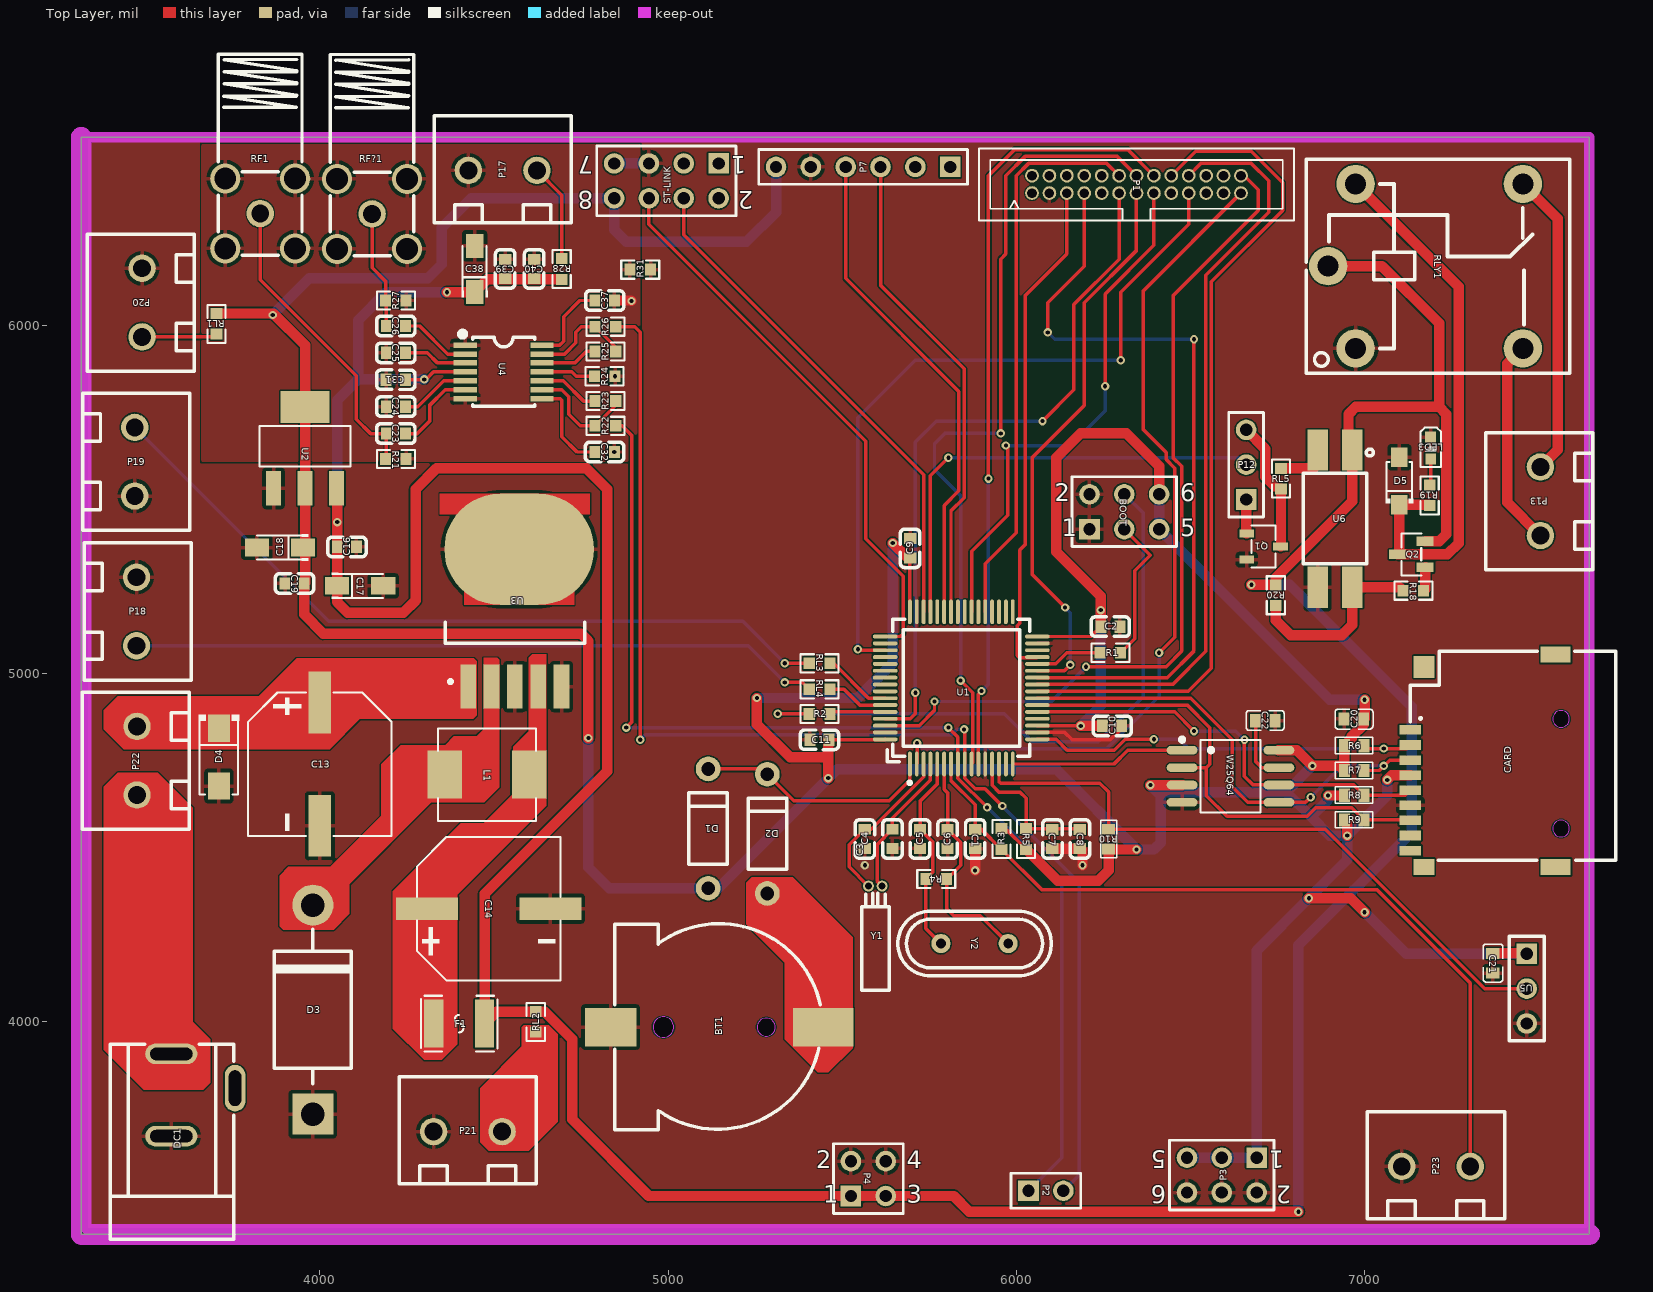
[diagram p0: Top Layer view]
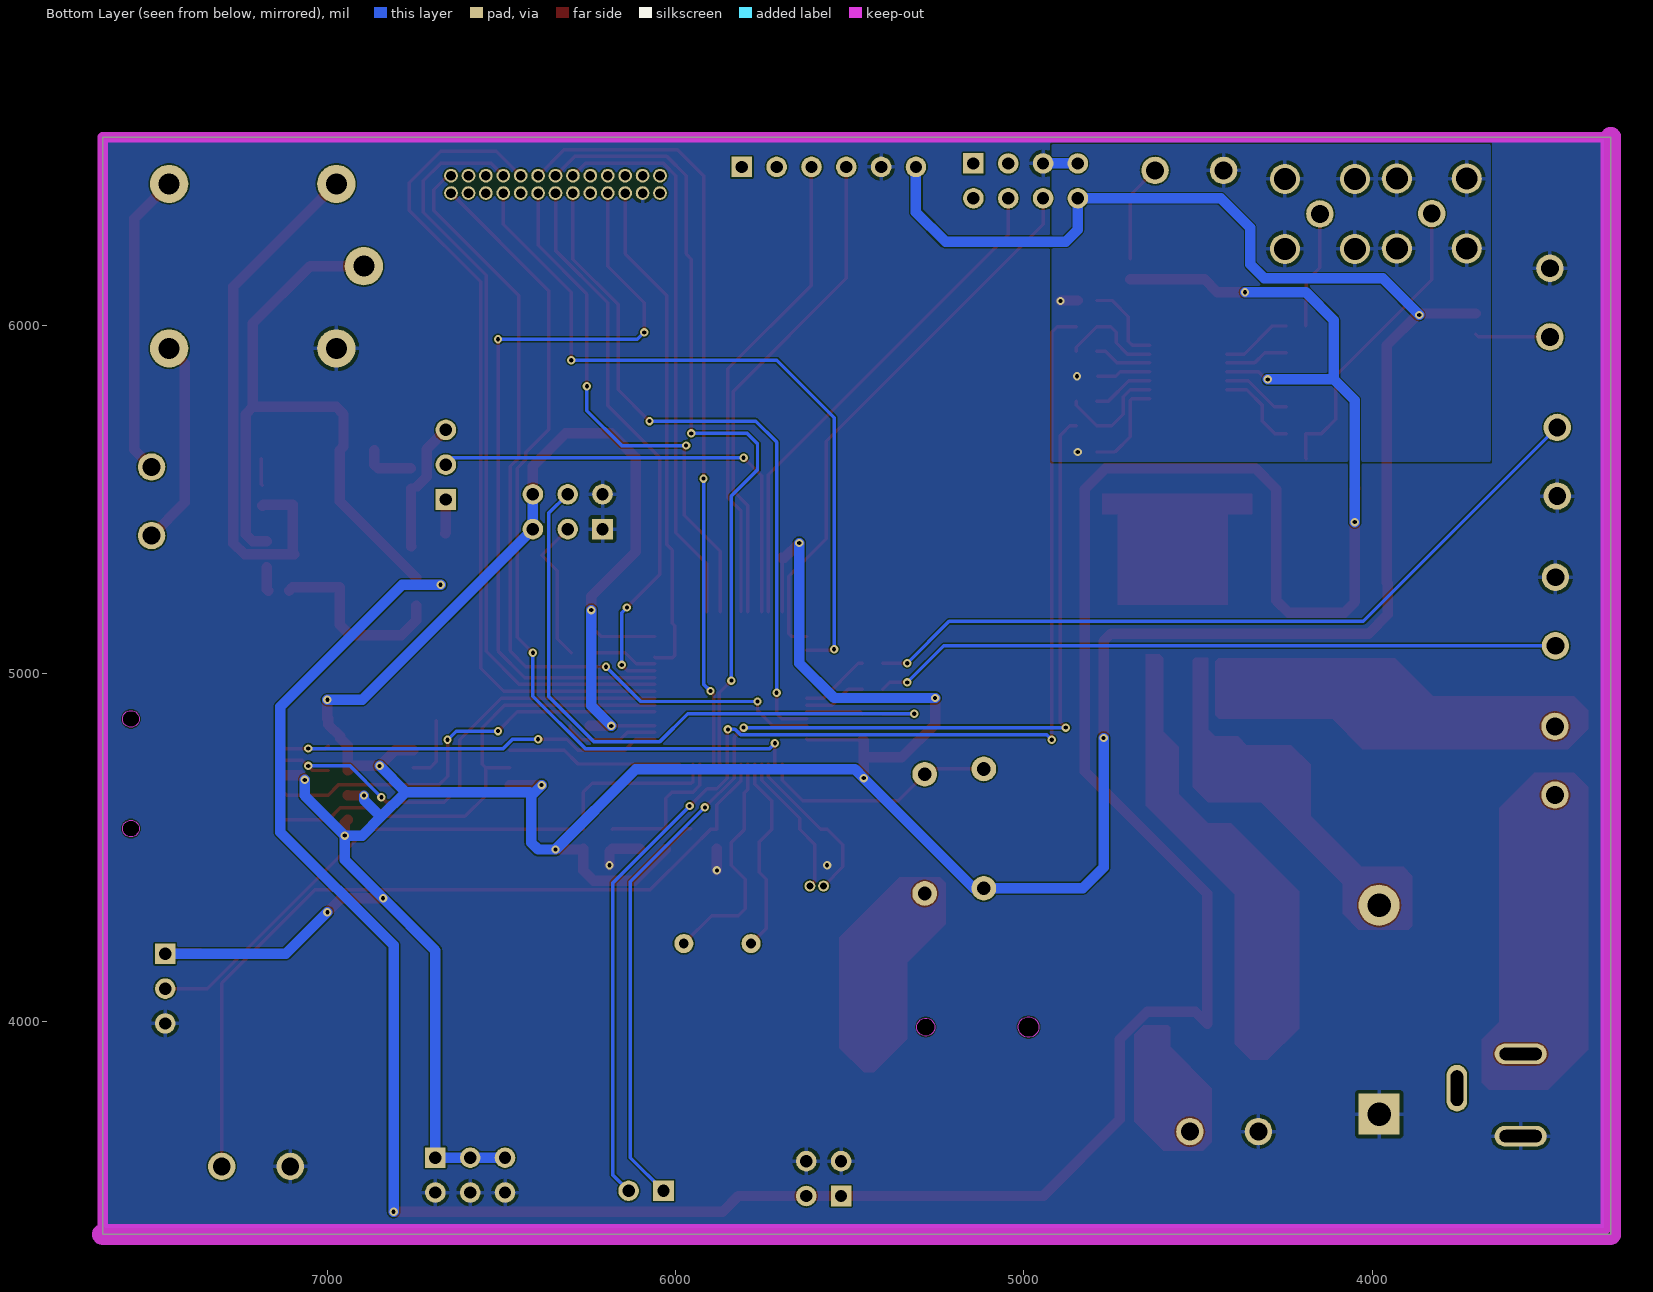
[diagram p1: Bottom Layer view, seen from below]
# Altium PCB MISC51485.pcbdoc
Units mil, origin at the board's own origin, x right, y up, seen from the top; angles counter-clockwise.
Board outline 4330.71 x 3150 mil, 2 copper layers (Top Layer, Bottom Layer); 98 components, 109 nets, 353 pads, 61 vias.

## Layer stack, top to bottom (the 12.6 mil dielectric is the usual default, probably not edited)
Top Solder Mask Layer: solder mask 0.4, Solder Resist, Dk 3.5
Top Layer: signal copper 1.4
Dielectric 1: surface 12.6, FR-4, Dk 4.8
Bottom Layer: signal copper 1.4
Bottom Solder Mask Layer: solder mask 0.4, Solder Resist, Dk 3.5

## Board outline
7645,3390 3315,3390 3315,6540 7645.71,6540 7645,6539.61

## Design rules (kind name [scope] priority, off if disabled: settings)
BoardOutlineClearance Clearance_1 [All] p2: genericclearance=4 ignorepadtopadclearanceinfootprint=FALSE except(0: Hole-OutlineEdge Arc-SplitContinuation Track-SplitContinuation SMDPad-SplitContinuation THPad-SplitContinuation Via-SplitContinuation Fill-SplitContinuation Region-SplitContinuation Poly-SplitContinuation Text-SplitContinuation Hole-SplitContinuation; 4: Arc-OutlineEdge Track-OutlineEdge SMDPad-OutlineEdge THPad-OutlineEdge Via-OutlineEdge Fill-OutlineEdge Region-OutlineEdge Poly-OutlineEdge Text-OutlineEdge Arc-CutoutEdge Track-CutoutEdge SMDPad-CutoutEdge THPad-CutoutEdge Poly-CutoutEdge; 6: Via-CutoutEdge Fill-CutoutEdge Region-CutoutEdge Text-CutoutEdge; 6.9: Hole-CutoutEdge)
Clearance [All] p1: gap=4 ignorepadtopadclearanceinfootprint=FALSE except(0: Hole-Track Hole-SMDPad Hole-THPad Hole-Via Fill-Hole Region-Hole Poly-Hole Hole-Arc Hole-Text)
DiffPairsRouting [All] p1: maxlimit=10 minlimit=6 mostfreqgap=6 toplayer_minwidth=15 toplayer_prefwidth=15 toplayer_maxwidth=15 toplayer_mingap=10 toplayer_prefgap=10 toplayer_maxgap=10 bottomlayer_minwidth=15 bottomlayer_prefwidth=15 bottomlayer_maxwidth=15 bottomlayer_mingap=10 bottomlayer_prefgap=10 bottomlayer_maxgap=10 maxuncoupledlength=10
HoleToHoleClearance ComponentClearance [All] p1: gap=10 allowstackedmicrovias=TRUE
Length netLength [All] p1: minlimit=0 maxlimit=0
MatchedLengths netLengthTolerance [All] p1: tolerance=1000
PolygonConnect [(InNet('AGND') OR InNet('GND'))] p1: connectstyle=Relief reliefconductorwidth=10 reliefentries=4 polygonreliefangle="90 Angle" airgapwidth=10 via.connectstyle=Relief via.reliefconductorwidth=10 via.reliefentries=4 via.polygonreliefangle="90 Angle" via.airgapwidth=10
RoutingVias [All] p1: holewidth=12 width=24 viastyle="Through Hole" minholewidth=1 minwidth=1 maxholewidth=28 maxwidth=50
SolderMaskExpansion [All] p1: expansion=4 istentingtop=FALSE
Width [All] p1: maxlimit=10 minlimit=10 preferedwidth=10 toplayer_minwidth=10 toplayer_maxwidth=300 toplayer_prefwidth=10 bottomlayer_minwidth=10 bottomlayer_maxwidth=300 bottomlayer_prefwidth=10
2 further rules are at their usual default settings.

## Components (designator, comment, footprint, x,y, rotation, side; value= is the part's Value field where it differs from the comment)
BOOT "Header 3X2" HDR2X3 6210,5415 r0 top
BT1 "BS-12-B3AA003" BAT-SMD_BS-12-B3AA011 5140,3985 r180 top
C1 "104" C0603 5881.72,4525 r270 top
C2 "104" C0603 6270,5135 r0 top
C3 "12pF" C0603 5644.23,4525.61 r90 top
C4 "12pF" C0603 5565,4525.61 r90 top
C5 "22pF" C0603 5723.46,4525.61 r90 top
C6 "22pF" C0603 5802.48,4525 r90 top
C7 "10uF" C0603 6103.2,4525 r270 top
C8 "104" C0603 6182.44,4525 r270 top
C9 "104" C0603 5695,5360 r90 top
C10 "104" C0603 6275,4850 r180 top
C11 "104" C0603 5435,4810 r0 top
C13 "GVM1V681M1010" CAP-SMD_BD10.0-L10.3-W10.3-LS10.9-FD 4000,4740 r270 top
C14 "EEEFK1V331P" CAP-SMD_BD10.0-L10.3-W10.3-FD 4485,4325 r0 top
C16 "104" C0603 4077.56,5363.94 r180 top
C17 "TAJA106K016RNJ" CAP-SMD_L3.2-W1.6-RD-C7171 4115.75,5252.05 r0 top
C18 "TAJA106K016RNJ" CAP-SMD_L3.2-W1.6-RD-C7171 3885.75,5362.17 r180 top
C19 "104" C0603 3927.56,5258.94 r0 top
C20 "Cap" CAP[0603] 6969.26,4869.85 r180 top
C21 "Cap" CAP[0603] 7368.1,4168.36 r270 top
C22 "Cap" CAP[0603] 6715,4865 r0 top
C23 "102" C0603 4218.55,5689.48 r0 top
C24 "102" C0603 4218.55,5766.66 r0 top
C25 "102" C0603 4218.55,5921.03 r0 top
C26 "102" C0603 4218.55,5998.21 r0 top
C31 "100pF" C0603 4217.94,5844.06 r180 top
C32 "0.1uF" C0603 4817.94,5636.45 r0 top
C37 "0.1uF" C0603 4817.94,6071.45 r180 top
C38 "10uF" CAP-SMD_L3.2-W1.6-RD-C7171 4444.5,6162.01 r90 top
C39 "0.1uF" C0603 4532.1,6161.7 r270 top
C40 "0.1uF" C0603 4615.28,6161.7 r270 top
CARD "TF PUSH" TF-SMD_TF-PUSH 7339.85,4749.85 r90 top
D1 "1N4733A_C5157516" DO-41_BD2.4-L4.7-P8.70-D0.9-RD 5115,4555 r270 top
D2 "1N4733A_C5157516" DO-41_BD2.4-L4.7-P8.70-D0.9-RD 5285,4540 r270 top
D3 "1N5822" DO-201AD_BD5.3-L8.4-P12.50-D1.4-FD 3980,4035 r90 top
D4 "1N4007_C727081" SMA_L4.3-W2.5-LS5.0-RD 3710,4760 r270 top
D5 "1N4007W" SOD-123FL_L2.7-W1.8-LS3.8-RD 7099.9,5553.14 r90 top
DC1 "DC-005-20A_C136744" DC-IN-TH_DC-005-20A 3665,3790 r90 top
F1 "BSMD1812-150-33V" F1812 4400,3995 r180 top
L1 "FXL0650-330-M" IND-SMD_L7.0-W6.6_FXL0650 4480,4710 r180 top
LED3 "NCD0603R1_C84263" LED0603-RD_RED 7189.87,5647.91 r270 top
P1 "X1270WV-2x13A-6TV01" IDC-TH_X1270WV-2X13A-6TV01 6345,6405 r0 top
P2 "Header 2" HDR1X2 6035,3515 r0 top
P3 "Header 3X2" HDR2X3 6690,3610 r180 top
P4 "Header 2X2" HDR2X2 5525,3500 r0 top
P7 "Header 6" HDR1X6 5810,6455 r180 top
P12 "Header 3" HDR1X3 6660,5500 r90 top
P13 "WJ126V-5.0-2P" CONN-TH_WJ126V-5.0-2P 7505,5495 r180 top
P17 "WJ126V-5.0-2P" CONN-TH_WJ126V-5.0-2P 4525,6445 r90 top
P18 "WJ126V-5.0-2P" CONN-TH_WJ126V-5.0-2P 3473.59,5178.49 r0 top
P19 "WJ126V-5.0-2P" CONN-TH_WJ126V-5.0-2P 3468.59,5608.49 r0 top
P20 "WJ126V-5.0-2P" CONN-TH_WJ126V-5.0-2P 3489.47,6065.51 r180 top
P21 "WJ126V-5.0-2P" CONN-TH_WJ126V-5.0-2P 4425,3685 r90 top
P22 "WJ126V-5.0-2P" CONN-TH_WJ126V-5.0-2P 3475,4750 r180 top
P23 "WJ126V-5.0-2P" CONN-TH_WJ126V-5.0-2P 7205,3585 r90 top
Q1 "DTC143ECA" SOT-23-3_L2.9-W1.6-P1.90-LS2.8-BR 6710,5365 r180 top
Q2 "MMBT3906" SOT-23-3_L2.9-W1.3-P1.90-LS2.4-BR 7134.21,5342.45 r0 top
R1 "10k" "R0603 - duplicate" 6270,5060 r0 top
R2 "10k" R0603 5435,4884.44 r0 top
R3 "10k" R0603 5957,4525.31 r90 top
R4 "1M" R0603 5770,4410 r180 top
R5 "10R" R0603 6028.13,4525.31 r270 top
R6 "Res" RES[0603] 6969.85,4792.85 r0 top
R7 "Res" RES[0603] 6969.85,4721.85 r0 top
R8 "Res" RES[0603] 6969.85,4650.85 r0 top
R9 "Res" RES[0603] 6969.85,4579.85 r0 top
R10 "Res" RES[0603] 6265,4525 r270 top
R18 "10k" "R0603 - duplicate" 7139.9,5238.14 r0 top
R19 "10k" "R0603 - duplicate" 7186.98,5511.83 r270 top
R20 "10k" "R0603 - duplicate" 6745,5225 r270 top
R21 "52.3R" R0603 4218.24,5616.45 r0 top
R22 "0" R0603 4820,5711.73 r180 top
R23 "100" R0603 4820,5782.84 r180 top
R24 "1K" R0603 4817.94,5853.95 r180 top
R25 "100" R0603 4820,5925.07 r180 top
R26 "0" R0603 4820,5996.18 r180 top
R27 "52.3R" R0603 4218.24,6071.45 r180 top
R28 "1K" R0603 4694.5,6162.01 r270 top
R31 "0" R0603 4920,6160 r180 top
RF1 "BWSMA-KWE-Z001" SMA-TH_BWSMA-KWE-Z001 3828.77,6321.23 r90 top
RF?1 "BWSMA-KWE-Z001" SMA-TH_BWSMA-KWE-Z001 4150,6320 r90 top
RL1 "330" "R0603 - duplicate" 3703.03,6004.51 r270 top
RL2 "330" "R0603 - duplicate" 4620,4000 r270 top
RL3 "330" "R0603 - duplicate" 5435,5029.72 r0 top
RL4 "330" "R0603 - duplicate" 5435,4955 r0 top
RL5 "330" "R0603 - duplicate" 6760,5560 r90 top
RLY1 "SRD-05VDC-SL-C" RELAY-TH_SRD-XXVDC-XL-C 7175,6170 r0 top
ST-LINK "Header 4X2" HDR2X4 5145,6465 r180 top
U1 "STM32F103RCT6" TQFP-64_L10.0-W10.0-P0.50-LS12.0-BL 5841.93,4959 r0 top
U2 "LM1117MPX-3.3/NOPB" SOT-223-3_L6.5-W3.4-P2.30-LS7.0-BR 3957.56,5648.94 r270 top
U3 "LM2596SX-5.0/NOPB" TO-263-5_L10.2-W8.9-P1.70-TL 4560,5160 r90 top
U4 "AD8302ARUZ-RL7" TSSOP-14_L5.0-W4.4-P0.65-LS6.4-BL 4527.94,5866.45 r270 top
U5 "DS18B20" H2.54-1X3(RM) 7465.79,4195.49 r270 top
U6 "BPC-817SC" OPTO-SMD-4_L4.6-W6.5-P2.54-LS10.3-BR 6915,5445 r90 top
W25Q64 "W25Q64JVSSIQ" SOIC-8_L5.3-W5.3-P1.27-LS8.0-BL 6615,4705.27 r270 top
Y1 "32.768kHz" OSC-TH_BD2.0-P0.70-D0.3 5595,4390 r90 top
Y2 "8MHz" OSC-TH_L11.1-W4.7-P4.88 5880,4225 r0 top

## Footprints (in the part's own frame and the unit in brackets; to place one, negate y for a bottom-side part, rotate by r counter-clockwise, add the part's x,y. Pads: shape width x height; smd on the part's side, far side on the other; paste and mask are expansions set on the pad)
BAT-SMD_BS-12-B3AA011 [mm]
  rect 3.75x2.8 smd: 1(7.75,0)
  rect 4.4x2.8 smd: 2(-7.75,0)
  Board Outline Layer lines w0.003: 4.649,0.098 4.65,0 4.649,-0.098 4.596,-0.287 4.497,-0.456 4.358,-0.594 4.187,-0.691 3.998,-0.741 3.802,-0.741 3.613,-0.691 3.443,-0.594 3.303,-0.456 3.204,-0.287 3.151,-0.098 3.15,0 3.151,0.098 3.204,0.287 3.303,0.456 3.443,0.594 3.613,0.691 3.802,0.741 3.998,0.741 4.188,0.691 4.358,0.594 4.497,0.456 4.596,0.287 4.649,0.098 ; -2.95,0.086 -2.95,0 -2.95,-0.086 -2.994,-0.251 -3.08,-0.399 -3.201,-0.52 -3.349,-0.606 -3.515,-0.65 -3.686,-0.65 -3.851,-0.606 -3.999,-0.52 -4.12,-0.399 -4.206,-0.251 -4.25,-0.086 -4.25,0 -4.25,0.086 -4.206,0.251 -4.12,0.399 -3.999,0.52 -3.851,0.606 -3.686,0.65 -3.514,0.65 -3.349,0.606 -3.201,0.52 -3.08,0.399 -2.994,0.251 -2.95,0.086
  Board Outline Layer region: -2.95,0 -2.95,0.086 -2.994,0.251 -3.08,0.399 -3.201,0.52 -3.349,0.606 -3.514,0.65 -3.686,0.65 -3.851,0.606 -3.999,0.52 -4.12,0.399 -4.206,0.251 -4.25,0.086 -4.25,0 -4.25,-0.086 -4.206,-0.251 -4.12,-0.399 -3.999,-0.52 -3.851,-0.606 -3.686,-0.65 -3.515,-0.65 -3.349,-0.606 -3.201,-0.52 -3.08,-0.399 -2.994,-0.251 -2.95,-0.086 -2.95,0 -2.95,0
  Board Outline Layer region: -2.95,0 -2.95,0.086 -2.994,0.251 -3.08,0.399 -3.201,0.52 -3.349,0.606 -3.514,0.65 -3.686,0.65 -3.851,0.606 -3.999,0.52 -4.12,0.399 -4.206,0.251 -4.25,0.086 -4.25,0 -4.25,-0.086 -4.206,-0.251 -4.12,-0.399 -3.999,-0.52 -3.851,-0.606 -3.686,-0.65 -3.515,-0.65 -3.349,-0.606 -3.201,-0.52 -3.08,-0.399 -2.994,-0.251 -2.95,-0.086 -2.95,0 -2.95,0
  Board Outline Layer region: -2.95,0 -2.95,0.086 -2.994,0.251 -3.08,0.399 -3.201,0.52 -3.349,0.606 -3.514,0.65 -3.686,0.65 -3.851,0.606 -3.999,0.52 -4.12,0.399 -4.206,0.251 -4.25,0.086 -4.25,0 -4.25,-0.086 -4.206,-0.251 -4.12,-0.399 -3.999,-0.52 -3.851,-0.606 -3.686,-0.65 -3.515,-0.65 -3.349,-0.606 -3.201,-0.52 -3.08,-0.399 -2.994,-0.251 -2.95,-0.086 -2.95,0 -2.95,0
  Board Outline Layer region: 4.65,0 4.649,0.098 4.596,0.287 4.497,0.456 4.358,0.594 4.188,0.691 3.998,0.741 3.802,0.741 3.613,0.691 3.443,0.594 3.303,0.456 3.204,0.287 3.151,0.098 3.15,0 3.151,-0.098 3.204,-0.287 3.303,-0.456 3.443,-0.594 3.613,-0.691 3.802,-0.741 3.998,-0.741 4.187,-0.691 4.358,-0.594 4.497,-0.456 4.596,-0.287 4.649,-0.098 4.65,0
  Board Outline Layer region: 4.65,0 4.649,0.098 4.596,0.287 4.497,0.456 4.358,0.594 4.188,0.691 3.998,0.741 3.802,0.741 3.613,0.691 3.443,0.594 3.303,0.456 3.204,0.287 3.151,0.098 3.15,0 3.151,-0.098 3.204,-0.287 3.303,-0.456 3.443,-0.594 3.613,-0.691 3.802,-0.741 3.998,-0.741 4.187,-0.691 4.358,-0.594 4.497,-0.456 4.596,-0.287 4.649,-0.098 4.65,0
  Board Outline Layer region: 4.65,0 4.649,0.098 4.596,0.287 4.497,0.456 4.358,0.594 4.188,0.691 3.998,0.741 3.802,0.741 3.613,0.691 3.443,0.594 3.303,0.456 3.204,0.287 3.151,0.098 3.15,0 3.151,-0.098 3.204,-0.287 3.303,-0.456 3.443,-0.594 3.613,-0.691 3.802,-0.741 3.998,-0.741 4.187,-0.691 4.358,-0.594 4.497,-0.456 4.596,-0.287 4.649,-0.098 4.65,0
  Multi-Layer board cut-out: -2.95,0 -2.95,0.086 -2.994,0.251 -3.08,0.399 -3.201,0.52 -3.349,0.606 -3.514,0.65 -3.686,0.65 -3.851,0.606 -3.999,0.52 -4.12,0.399 -4.206,0.251 -4.25,0.086 -4.25,0 -4.25,-0.086 -4.206,-0.251 -4.12,-0.399 -3.999,-0.52 -3.851,-0.606 -3.686,-0.65 -3.515,-0.65 -3.349,-0.606 -3.201,-0.52 -3.08,-0.399 -2.994,-0.251 -2.95,-0.086 -2.95,0 -2.95,0
  Multi-Layer board cut-out: 4.65,0 4.649,0.098 4.596,0.287 4.497,0.456 4.358,0.594 4.188,0.691 3.998,0.741 3.802,0.741 3.613,0.691 3.443,0.594 3.303,0.456 3.204,0.287 3.151,0.098 3.15,0 3.151,-0.098 3.204,-0.287 3.303,-0.456 3.443,-0.594 3.613,-0.691 3.802,-0.741 3.998,-0.741 4.187,-0.691 4.358,-0.594 4.497,-0.456 4.596,-0.287 4.649,-0.098 4.65,0
  silkscreen extent -7.55,-7.54 7.44,7.49
C0603 [mm]
  rect 0.8x0.9 smd paste+0 mask+0.051: 1(-0.7,0) 2(0.7,0)
  silkscreen extent -1.41,-0.71 1.39,0.72
CAP-SMD_BD10.0-L10.3-W10.3-FD [mm]
  rect 4.5x1.65 smd: 1(-4.5,0) 2(4.5,0)
  silkscreen extent -5.23,-5.23 5.23,5.23
CAP-SMD_BD10.0-L10.3-W10.3-LS10.9-FD [mm]
  rect 4.5x1.65 smd: 1(-4.5,0) 2(4.5,0)
  silkscreen extent -5.23,-5.23 5.23,5.23
CAP-SMD_L3.2-W1.6-RD-C7171 [mil]
  rect 69.19x51.02 smd: 1(-66.39,0) 2(66.39,0)
  silkscreen extent -81,-37 66,37
CAP[0603] [mm]
  rect 0.8x0.965 smd: 1(-0.716,0) 2(0.716,0)
  silkscreen extent -1.4,-0.71 1.37,0.74
CONN-TH_WJ126V-5.0-2P [mm]
  round 2 hole 1.3: 1(0,2.501) 2(0,-2.501)
  silkscreen extent -3.8,-5 4,5
DC-IN-TH_DC-005-20A [mm]
  oval 1.5x3.8 hole 0.9 slot 3.1 at 90 deg copper offset 0.001,0 paste+0 mask+0.051: 1(2.999,2.325)
  oval 1.5x3.8 hole 0.9 slot 3.1 at 90 deg copper offset 0,0 paste+0 mask+0.051: 2(-3.001,2.325)
  oval 3.4x1.5 hole 0.9 slot 2.6 at 0 deg copper offset 0.001,0 paste+0 mask+0.051: 3(0.5,-2.326)
  silkscreen extent -10.51,-2.24 3.71,6.78
DO-41_BD2.4-L4.7-P8.70-D0.9-RD [mm]
  round 1.8 hole 1: 1(-4.35,0) 2(4.35,0)
  silkscreen extent -2.6,-1.4 2.6,1.4
DO-201AD_BD5.3-L8.4-P12.50-D1.4-FD [mm]
  rect 3x3 hole 1.7: 1(-7.62,0)
  round 3 hole 1.7: 2(7.62,0)
  silkscreen extent -5.39,-2.8 5.87,2.8
F1812 [mil]
  rect 55.38x137.76 smd paste-3937.01 mask+2: 1(-72.97,0) 2(72.97,0)
  silkscreen extent -110,-80 110,80
H2.54-1X3(RM) [mm]
  rect 1.5x1.5 hole 0.9: 1(0,0)
  round 1.5 hole 0.9: 2(2.54,0) 3(5.08,0)
  silkscreen extent -1.27,-1.27 6.35,1.27
HDR1X2 [mm]
  rect 1.5x1.5 hole 0.9: 1(0,0)
  round 1.5 hole 0.9: 2(2.54,0)
  silkscreen extent -1.27,-1.27 3.81,1.27
HDR1X3 [mm]
  rect 1.5x1.5 hole 0.9: 1(0,0)
  round 1.5 hole 0.9: 2(2.54,0) 3(5.08,0)
  silkscreen extent -1.27,-1.27 6.35,1.27
HDR1X6 [mm]
  rect 1.5x1.5 hole 0.9: 1(0,0)
  round 1.5 hole 0.9: 2(2.54,0) 3(5.08,0) 4(7.62,0) 5(10.16,0) 6(12.7,0)
  silkscreen extent -1.27,-1.27 13.97,1.27
HDR2X2 [mm]
  rect 1.5x1.5 hole 0.9: 1(0,0)
  round 1.5 hole 0.9: 2(0,2.54) 3(2.54,0) 4(2.54,2.54)
  silkscreen extent -1.27,-1.27 3.81,3.81
HDR2X3 [mm]
  rect 1.5x1.5 hole 0.9: 1(0,0)
  round 1.5 hole 0.9: 2(0,2.54) 3(2.54,0) 4(2.54,2.54) 5(5.08,0) 6(5.08,2.54)
  silkscreen extent -1.27,-1.27 6.35,3.81
HDR2X4 [mm]
  rect 1.5x1.5 hole 0.9: 1(0,0)
  round 1.5 hole 0.9: 2(0,2.54) 3(2.54,0) 4(2.54,2.54) 5(5.08,0) 6(5.08,2.54) 7(7.62,0) 8(7.62,2.54)
  silkscreen extent -1.27,-1.27 8.89,3.81
IDC-TH_X1270WV-2X13A-6TV01 [mm]
  round 1 hole 0.7 paste+0 mask+0.05: 1(-7.62,-0.635) 2(-7.62,0.635) 3(-6.35,-0.635) 4(-6.35,0.635) 5(-5.08,-0.635) 6(-5.08,0.635) 7(-3.81,-0.635) 8(-3.81,0.635) 9(-2.54,-0.635) 10(-2.54,0.635) 11(-1.27,-0.635) 12(-1.27,0.635) 13(0,-0.635) 14(0,0.635) 15(1.27,-0.635) 16(1.27,0.635) 17(2.54,-0.635) 18(2.54,0.635) 19(3.81,-0.635) 20(3.81,0.635) 21(5.08,-0.635) 22(5.08,0.635) 23(6.35,-0.635) 24(6.35,0.635) 25(7.62,-0.635) 26(7.62,0.635)
  silkscreen extent -11.48,-2.63 11.48,2.63
IND-SMD_L7.0-W6.6_FXL0650 [mm]
  rect 2.524x3.5 smd: 1(3.078,0) 2(-3.078,0)
  silkscreen extent -3.58,-3.38 3.58,3.38
LED0603-RD_RED [mm]
  rect 0.8x0.8 smd: 1(-0.8,-0.003) 2(0.8,0.003)
  silkscreen extent -1.49,-0.75 1.39,0.76
OPTO-SMD-4_L4.6-W6.5-P2.54-LS10.3-BR [mm]
  rect 3x1.5 smd: 1(5,-1.27) 2(5,1.27) 3(-5,1.27) 4(-5,-1.27)
  silkscreen extent -3.3,-2.79 5.08,2.3
OSC-TH_BD2.0-P0.70-D0.3 [mm]
  round 0.8 hole 0.5 paste+0 mask+0.051: 1(0,0.5) 2(0,-0.5)
  silkscreen extent -7.6,-1 -0.54,1
OSC-TH_L11.1-W4.7-P4.88 [mm]
  round 1.4 hole 0.7 paste+0 mask+0.051: 1(-2.45,0) 2(2.45,0)
  silkscreen extent -5.59,-2.35 5.6,2.35
R0603 [mil]
  rect 31.75x34.02 smd paste+0 mask+2: 1(-29.66,0) 2(29.66,0)
  silkscreen extent -55,-26 55,26
"R0603 - duplicate" [mil]
  rect 31.75x34.02 smd paste+0 mask+2: 1(-29.66,0) 2(29.66,0)
  silkscreen extent -55,-26 55,26
RELAY-TH_SRD-XXVDC-XL-C [mil]
  round 110 hole 60: 1(-200.79,-236.22) 2(279.52,-236.2) 3(279.53,236.2) 4(-200.79,236.22) 5(-279.53,0)
  silkscreen extent -342,-307 413,307
RES[0603] [mm]
  rect 0.8x0.965 smd: 1(-0.716,0) 2(0.716,0)
  silkscreen extent -1.37,-0.58 1.37,0.61
SMA-TH_BWSMA-KWE-Z001 [mm]
  round 2.2 hole 1.6: 1(-2.55,-2.55) 2(-2.55,2.55) 3(2.55,2.55)
  round 2.2 hole 1.6 copper offset 0,0: 4(2.55,-2.55)
  round 2 hole 1.3: 5(0,0)
  silkscreen extent -3.05,-3.05 11.63,3.05
SMA_L4.3-W2.5-LS5.0-RD [mm]
  rect 2x1.593 smd: 1(-2.1,0) 2(2.1,0)
  silkscreen extent -3.11,-1.48 2.73,1.48
SOD-123FL_L2.7-W1.8-LS3.8-RD [mm]
  rect 1.4x1.2 smd: 1(-1.735,0) 2(1.735,0)
  silkscreen extent -1.6,-1 1.38,1
SOIC-8_L5.3-W5.3-P1.27-LS8.0-BL [mm]
  oval 0.63x2.25 smd: 1(-1.905,-3.53) 2(-0.635,-3.53) 3(0.635,-3.53) 4(1.905,-3.53) 5(1.905,3.53) 6(0.635,3.53) 7(-0.635,3.53) 8(-1.905,3.53)
  silkscreen extent -2.82,-3.68 2.64,2.18
SOT-23-3_L2.9-W1.3-P1.90-LS2.4-BR [mm]
  rect 1.25x0.7 smd paste+0 mask+0.051: 1(1,-0.95) 2(1,0.95) 3(-1,0)
  silkscreen extent -0.73,-1.53 0.73,1.53
SOT-23-3_L2.9-W1.6-P1.90-LS2.8-BR [mm]
  rect 1.07x0.6 smd paste+0 mask+0.051: 1(1.235,-0.95) 2(1.235,0.95) 3(-1.235,0)
  silkscreen extent -0.88,-1.54 0.88,1.54
SOT-223-3_L6.5-W3.4-P2.30-LS7.0-BR [mm]
  rect 2.5x1.1 smd paste+0 mask+0.051: 1(2.97,-2.3) 2(2.97,0) 3(2.97,2.3)
  rect 2.34x3.6 smd paste+0 mask+0.051: 4(-2.97,0)
  silkscreen extent -1.57,-3.33 1.37,3.33
TF-SMD_TF-PUSH [mm]
  rect 0.7x1.6 smd: 1(2.25,5.3) 2(1.15,5.3) 3(0.05,5.3) 4(-1.05,5.3) 5(-2.15,5.3) 6(-3.25,5.3) 7(-4.35,5.3) 8(-5.45,5.3) CD(-6.55,5.3)
  rect 1.2x1.5 smd: 10(-7.75,4.3)
  rect 1.2x2.2 smd: 11(-7.75,-5.3) 12(7.75,-5.3)
  rect 1.6x1.5 smd: 13(6.85,4.3)
  Board Outline Layer lines w0.003: -5.069,-5.1 -4.831,-5.1 -4.61,-5.191 -4.441,-5.36 -4.35,-5.581 -4.35,-5.7 -4.35,-5.819 -4.441,-6.04 -4.61,-6.209 -4.831,-6.3 -5.069,-6.3 -5.29,-6.209 -5.459,-6.04 -5.55,-5.819 -5.55,-5.7 -5.55,-5.581 -5.459,-5.36 -5.29,-5.191 -5.069,-5.1 ; 2.931,-5.1 3.169,-5.1 3.39,-5.191 3.559,-5.36 3.65,-5.581 3.65,-5.7 3.65,-5.819 3.559,-6.04 3.39,-6.209 3.169,-6.3 2.931,-6.3 2.71,-6.209 2.541,-6.04 2.45,-5.819 2.45,-5.7 2.45,-5.581 2.541,-5.36 2.71,-5.191 2.931,-5.1
  Board Outline Layer region: 3.65,-5.7 3.65,-5.581 3.559,-5.36 3.39,-5.191 3.169,-5.1 2.931,-5.1 2.71,-5.191 2.541,-5.36 2.45,-5.581 2.45,-5.7 2.45,-5.819 2.541,-6.04 2.71,-6.209 2.931,-6.3 3.169,-6.3 3.39,-6.209 3.559,-6.04 3.65,-5.819
  Board Outline Layer region: 3.65,-5.7 3.65,-5.581 3.559,-5.36 3.39,-5.191 3.169,-5.1 2.931,-5.1 2.71,-5.191 2.541,-5.36 2.45,-5.581 2.45,-5.7 2.45,-5.819 2.541,-6.04 2.71,-6.209 2.931,-6.3 3.169,-6.3 3.39,-6.209 3.559,-6.04 3.65,-5.819
  Board Outline Layer region: -4.35,-5.7 -4.35,-5.581 -4.441,-5.36 -4.61,-5.191 -4.831,-5.1 -5.069,-5.1 -5.29,-5.191 -5.459,-5.36 -5.55,-5.581 -5.55,-5.7 -5.55,-5.819 -5.459,-6.04 -5.29,-6.209 -5.069,-6.3 -4.831,-6.3 -4.61,-6.209 -4.441,-6.04 -4.35,-5.819
  Board Outline Layer region: -4.35,-5.7 -4.35,-5.581 -4.441,-5.36 -4.61,-5.191 -4.831,-5.1 -5.069,-5.1 -5.29,-5.191 -5.459,-5.36 -5.55,-5.581 -5.55,-5.7 -5.55,-5.819 -5.459,-6.04 -5.29,-6.209 -5.069,-6.3 -4.831,-6.3 -4.61,-6.209 -4.441,-6.04 -4.35,-5.819
  Multi-Layer board cut-out: 3.65,-5.7 3.65,-5.581 3.559,-5.36 3.39,-5.191 3.169,-5.1 2.931,-5.1 2.71,-5.191 2.541,-5.36 2.45,-5.581 2.45,-5.7 2.45,-5.819 2.541,-6.04 2.71,-6.209 2.931,-6.3 3.169,-6.3 3.39,-6.209 3.559,-6.04 3.65,-5.819
  Multi-Layer board cut-out: -4.35,-5.7 -4.35,-5.581 -4.441,-5.36 -4.61,-5.191 -4.831,-5.1 -5.069,-5.1 -5.29,-5.191 -5.459,-5.36 -5.55,-5.581 -5.55,-5.7 -5.55,-5.819 -5.459,-6.04 -5.29,-6.209 -5.069,-6.3 -4.831,-6.3 -4.61,-6.209 -4.441,-6.04 -4.35,-5.819
  silkscreen extent -7.26,-9.7 8,5.3
TO-263-5_L10.2-W8.9-P1.70-TL [mm]
  rect 3.2x1.15 smd: 1(-5.008,3.404) 2(-5.008,1.702) 3(-5.008,0) 4(-5.008,-1.702) 5(-5.008,-3.404)
  oval 8.128x10.922 smd: 6(5.008,-0.317)
  Top Layer region: 0.944,3.683 7.548,3.683 7.548,5.461 9.072,5.461 9.072,-5.461 7.548,-5.461 7.548,-4.317 0.944,-4.317
  silkscreen extent -4.77,-5.08 -0.33,5.08
TQFP-64_L10.0-W10.0-P0.50-LS12.0-BL [mm]
  oval 0.28x1.8 smd paste+0 mask+0.051: 1(-3.75,-5.55) 2(-3.25,-5.55) 3(-2.75,-5.55) 4(-2.25,-5.55) 5(-1.75,-5.55) 6(-1.25,-5.55) 7(-0.75,-5.55) 8(-0.25,-5.55) 9(0.25,-5.55) 10(0.75,-5.55) 11(1.25,-5.55) 12(1.75,-5.55) 13(2.25,-5.55) 14(2.75,-5.55) 15(3.25,-5.55) 16(3.75,-5.55) 33(3.75,5.55) 34(3.25,5.55) 35(2.75,5.55) 36(2.25,5.55) 37(1.75,5.55) 38(1.25,5.55) 39(0.75,5.55) 40(0.25,5.55) 41(-0.25,5.55) 42(-0.75,5.55) 43(-1.25,5.55) 44(-1.75,5.55) 45(-2.25,5.55) 46(-2.75,5.55) 47(-3.25,5.55) 48(-3.75,5.55)
  oval 1.8x0.28 smd paste+0 mask+0.051: 17(5.55,-3.75) 18(5.55,-3.25) 19(5.55,-2.75) 20(5.55,-2.25) 21(5.55,-1.75) 22(5.55,-1.25) 23(5.55,-0.75) 24(5.55,-0.25) 25(5.55,0.25) 26(5.55,0.75) 27(5.55,1.25) 28(5.55,1.75) 29(5.55,2.25) 30(5.55,2.75) 31(5.55,3.25) 32(5.55,3.75) 49(-5.55,3.75) 50(-5.55,3.25) 51(-5.55,2.75) 52(-5.55,2.25) 53(-5.55,1.75) 54(-5.55,1.25) 55(-5.55,0.75) 56(-5.55,0.25) 57(-5.55,-0.25) 58(-5.55,-0.75) 59(-5.55,-1.25) 60(-5.55,-1.75) 61(-5.55,-2.25) 62(-5.55,-2.75) 63(-5.55,-3.25) 64(-5.55,-3.75)
  silkscreen extent -5.4,-7.04 5,5
TSSOP-14_L5.0-W4.4-P0.65-LS6.4-BL [mm]
  rect 0.4x1.7 smd: 1(-1.95,-2.8) 2(-1.3,-2.8) 3(-0.65,-2.8) 4(0,-2.8) 5(0.65,-2.8) 6(1.3,-2.8) 7(1.95,-2.8) 8(1.95,2.8) 9(1.3,2.8) 10(0.65,2.8) 11(0,2.8) 12(-0.65,2.8) 13(-1.3,2.8) 14(-1.95,2.8)
  silkscreen extent -2.95,-3.2 2.5,2.25

## Via types
v1: diameter 24.02, hole 12, Top Layer to Bottom Layer, 61 vias

## Nets (pads, with @x,y where several pads share a name; then routed paths per layer and width w, separated by ;. In a path a pad name is that pad's centre, name@x,y a point inside that pad or via, vN(x,y) a via of type N, cw(c..) or ccw(c..) an arc to the next point about the centre after c; other vN are vias at no path point)
18B20_DQ: R10.1 U1.14 U5.2 | length 1875
  Top Layer w10: U1.14 5950.2,4689.8 5955,4685 6240,4685 6265,4660 R10.1 6886.81,4553.19 7344.51,4095.49 U5.2
$2N134: C6.2 R4.1 U1.6 Y2.2 | length 669.8
  Top Layer w10: U1.6 5792.72,4667.28 5802.48,4657.52 C6.2 5840,4515.04 5840,4450.34 R4.1 5799.66,4325.34 5820,4305 5896.45,4305 Y2.2
$2N135: C5.2 R4.2 U1.5 Y2.1 | length 577.2
  Top Layer w10: U1.5 5773.03,4683.03 5723.46,4633.46 C5.2 5760,4516.63 5760,4429.66 R4.2 5740.34,4268.21 Y2.1@5783.55,4225
$2N136: C7.1 C8.1 R5.1 U1.13 | length 416.4
  Top Layer w10: U1.13 5930.51,4679.49 5950,4660 6010,4660 6028.13,4641.87 R5.1 6180.03,4554.97 C8.1
$2N137: C4.2 U1.3 Y1.1 | length 472.6
  Top Layer w10: Y1.1 5520,4445.31 5520,4508.17 C4.2 5583.17,4553.17 5733.66,4703.66 U1.3
$2N138: C3.2 U1.4 Y1.2 | length 420.1
  Top Layer w10: Y1.2 5600,4404.69 5600,4508.94 C3.2 5644.23,4584.23 5753.35,4693.35 U1.4
$2N139: ST-LINK.2
$2N140: BOOT.3 R1.2 | length 421.4
  Top Layer w10: R1.2 6340,5100.34 6340,5295 6385,5340 BOOT.3
$2N141: BOOT.4 R2.1 | length 1830.3
  Top Layer w10: v1(5315,4885) 5315.56,4884.44 R2.1
  Bottom Layer w10: v1(5315,4885) 5965,4885 6045,4805 6235,4805 6365,4935 6365,5460 BOOT.4
$2N142: P20.1 RL1.2 | length 216.8
  Top Layer w10: P20.1 3695.24,5967.06 RL1.2
$2N143: P7.1
$2N144: P7.2
$2N145: P1.23
$2N146: P1.21
$2N147: P1.17
$2N148: P1.9
$2N149: P1.1
$2N150: P1.24
$2N151: P1.22
$2N152: P1.10
$2N153: P1.8
$2N154: P1.6
$2N155: P1.4
$2N156: P1.2
$2N157: D1.1 D2.1 U1.1 | length 687.9
  Top Layer w10: D1.1 5270,4726.26 D2.1 5361.26,4635 5635,4635 5694.29,4694.29 U1.1
$2N158: BT1.2 D2.2
$2N159: C22.1 W25Q64.7 | length 191.4
  Top Layer w10: C22.1 6686.81,4748.19 6704.73,4730.27 W25Q64.7
$2N160: D3.2 L1.1 U3.2
$2N161: C14.1 F1.2 L1.2 U3.4
$2N162: C13.1 D4.1 P22.2 U3.1
$2N163: P19.1 RL3.1 | length 2217.3
  Top Layer w10: v1(5335,5030) 5405.06,5030 RL3.1
  Bottom Layer w10: P19.1 4025.53,5150 5215,5150 v1(5335,5030)
$2N164: P18.2 RL4.1 | length 1983.5
  Top Layer w10: v1(5335,4975) 5385.34,4975 RL4.1
  Bottom Layer w10: P18.2 5229.96,5080.04 v1(5335,4975)
$2N165: P21.2 RL2.2
$3N29: C32.1 U4.8 | length 277.2
  Top Layer w10: U4.8 4690.32,5789.68 4695,5785 4695,5680 4738.55,5636.45 C32.1
$3N30: R23.2 U4.10 | length 176.2
  Top Layer w10: U4.10 4699.14,5840.86 4757.16,5782.84 R23.2
$3N31: R22.2 R23.1 U4.9 | length 320
  Top Layer w10: U4.9 4694.73,5815.27 4715,5795 4715,5745 4748.27,5711.73 R22.2 4849.66,5771.05 R23.1
$3N32: R25.2 U4.12 | length 165.8
  Top Layer w10: U4.12 4732.04,5892.04 4765.07,5925.07 R25.2
$3N33: R25.1 R26.2 U4.13 | length 298
  Top Layer w10: U4.13 4702.63,5917.63 4735,5950 4735,5980 4751.18,5996.18 R26.2 4849.66,5936.86 R25.1
$3N34: C26.1 R27.2 RF?1.5 | length 338.8
  Top Layer w10: RF?1.5 4149.99,6165.01 4188.58,6126.42 R27.2 4190.99,6069.05 C26.1
$3N35: C23.1 R21.1 RF1.5 | length 882.4
  Top Layer w10: RF1.5 3828.76,6131.24 4105,5855 4105,5730 4145.52,5689.48 C23.1 4190.99,5618.86 R21.1
$3N36: P17.2 R28.1 | length 282.8
  Top Layer w10: P17.2 4694.5,6373.95 R28.1
$3N37: R24.2 U4.11 | length 155.3
  Top Layer w10: U4.11 4723.55,5866.45 4736.05,5853.95 R24.2
$3N38: C37.2 U4.14 | length 246.3
  Top Layer w10: U4.14 4688.22,5943.22 4700,5955 4700,6025 4746.45,6071.45 C37.2
$3N39: C24.2 U4.5 | length 202.3
  Top Layer w10: C24.2 4281.66,5766.66 4355.86,5840.86 U4.5
$3N40: C25.2 U4.3 | length 183.6
  Top Layer w10: C25.2 4308.97,5921.03 4337.96,5892.04 U4.3
$3N41: C23.2 U4.6 | length 250.1
  Top Layer w10: C23.2 4279.48,5689.48 4315,5725 4315,5770 4360.27,5815.27 U4.6
$3N42: C26.2 U4.2 | length 205
  Top Layer w10: C26.2 4286.79,5998.21 4367.37,5917.63 U4.2
$3N43: P12.1 Q1.1 | length 98.2
  Top Layer w30: P12.1 6660,5403.77 Q1.1
$3N44: P12.3 Q1.3 RL5.1 | length 362.3
  Top Layer w30: P12.3 6715,5645 6715,5565 6742.33,5537.67 ; Q1.3 6760,5366.38 RL5.1
$3N45: RL5.2 U6.2 | length 151.1
  Top Layer w30: RL5.2 6854.66,5589.66 6865,5600 U6.2
$3N46: R18.1 R20.2 U6.4 | length 550.2
  Top Layer w30: R20.2 6745,5152.91 6787.91,5110 6935,5110 6965,5140 U6.4 7100.23,5248.15 R18.1
$3N47: Q2.1 R18.2 | length 68.6
  Top Layer w30: R18.2 7173.58,5242.16 Q2.1
$3N48: D5.1 Q2.3 R19.2 RLY1.4 | length 1575
  Top Layer w30: RLY1.4 7270,6110.43 7270,5375 7237.45,5342.45 Q2.3 7099.9,5347.51 D5.1 7184.32,5484.83 R19.2
$3N49: P13.2 RLY1.3 | length 875.1
  Top Layer w30: RLY1.3 7555,6305.73 7555,5643.45 P13.2
$3N50: P13.1 RLY1.2 | length 595
  Top Layer w30: RLY1.2 7410,5889.27 7410,5491.55 P13.1
$3N51: LED3.2 R19.1 | length 76.2
  Top Layer w10: R19.1 7190,5544.51 LED3.2
AGND: BOOT.1 BOOT.2 BT1.1 C1.2 C2.2 C3.1 C4.1 C5.1 C6.1 C7.2 C8.2 C9.2 C10.1 C11.1 C13.2 C14.2 C16.1 C17.2 C18.2 C19.1 C20.2 C21.2 C22.2 CARD.6 D3.1 D4.2 D5.2 DC1.2 LED3.1 P1.3 P3.2 P3.4 P3.6 P4.2 P4.4 P7.5 P18.1 P19.2 P20.2 P21.1 P23.1 Q1.2 R31.1 RLY1.1 ST-LINK.5 ST-LINK.7 U1.12 U1.18 U1.31 U1.47 U1.63 U2.1 U3.3 U3.5 U3.6 U5.3 U6.3 W25Q64.4 | length 564
  Top Layer w10: U1.18 6138.95,4831.05 6160,4810 6270,4810 6302.56,4842.56 C10.1
  Top Layer w30: v1(5881.72,4435) C1.2 ; C7.2 C8.2 6190,4489.88 v1(6190,4450)
  Bottom Layer w30: ST-LINK.7 ST-LINK.5
  other v1: 5565,4450
AVDD3.3: BOOT.5 BOOT.6 C2.1 C9.1 C10.2 C11.2 C18.1 C19.2 C20.1 C21.1 CARD.4 D1.2 P3.1 P3.3 P3.5 P7.6 R3.2 R5.2 R6.1 R7.1 R8.1 R9.1 R10.2 RL1.1 ST-LINK.8 U1.19 U1.32 U1.48 U1.64 U2.2 U2.4 U5.1 W25Q64.3 W25Q64.8 | length 14994.4
  Top Layer w10: C11.2 5622.07,4810 U1.64 ; U1.48 5694.29,5331.73 C9.1 ; R3.2 5968.81,4554.97 R5.2 ; U1.19 6184.27,4850.73 v1(6185,4850) ; U1.32 6214.08,5106.64 C2.1
  Top Layer w30: RL1.1 3865.83,6034.17 3957.56,5942.44 U2.4 U2.2 3957.56,5261.38 C19.2 3955.12,5169.88 4010,5115 4750,5115 4771.21,5093.79 v1(4771.21,4815) ; v1(5255,4930) 5255,4855 5350.25,4759.75 5460,4759.75 ; v1(5460,4700) 5460,4759.75 ; C11.2 5460,4807.44 5460,4759.75 ; v1(5645,5375) 5687.56,5332.44 C9.1 ; R5.2 6118.77,4405 6235,4405 6265,4435 R10.2 6266.81,4495 v1(6345,4495) ; v1(6185,4850) C10.2 ; C2.1 v1(6242.44,5182.49) 6242.44,5222.56 6115,5350 6115,5620 6184.9,5689.9 6315.1,5689.9 6410,5595 BOOT.6 ; v1(6385,4680) 6475.75,4680 W25Q64.3 ; W25Q64.8 6804.73,4780.27 v1(6850,4735) 6928.51,4735 R7.1 R6.1 6963.29,4814.48 6963.29,4819.72 6997.45,4853.87 C20.1 7000,4872.41 v1(7000,4925) ; v1(6840,4355) 6960,4355 v1(7000,4315) ; v1(6895,4650) 6940.81,4650 R8.1 ; R9.1 6950,4571.51 v1(6950,4535) ; v1(7065,4695) 7078.51,4708.51 CARD.4 ; C21.1 7464.73,4196.55 U5.1
  Bottom Layer w30: v1(3865,6030) 3970,6135 4310,6135 4350,6175 4350,6280 4435,6365 ST-LINK.8 4845,6275 4880,6240 5225,6240 5310,6325 P7.6 ; v1(4771.21,4815) 4771.21,4443.79 4831.26,4383.74 D1.2 5143.74,4383.74 v1(5460,4700) 5485,4725 6115,4725 v1(6345,4495) 6395,4495 6415,4515 6415,4650 v1(6385,4680) ; v1(5255,4930) 5545,4930 5645,5030 v1(5645,5375) ; v1(6185,4850) 6242.44,4907.44 v1(6242.44,5182.49) ; BOOT.6 BOOT.5 6900,4925 v1(7000,4925) ; 6420,4660 6775,4660 ; P3.5 P3.3 P3.1 6690,4205 v1(6840,4355) 6950,4465 v1(6950,4535) ; v1(6850,4735) 6775,4660 ; v1(6895,4650) 6895,4637.47 6846.27,4588.73 ; v1(7000,4315) 7119.51,4195.49 U5.1 ; v1(7065,4695) 7065,4650 v1(6950,4535) ; 6775,4660 6846.27,4588.73 ; 6846.27,4588.73 6900,4535 v1(6950,4535)
BOOT0: R2.2 U1.60 | length 161.1
  Top Layer w10: R2.2 5470.32,4890.1 U1.60
BOOT1: R1.1 U1.28 | length 193.2
  Top Layer w10: U1.28 6112.9,5027.9 6145,5060 R1.1
F_CS: U1.16 W25Q64.1 | length 502.9
  Top Layer w10: U1.16 6280.5,4740.5 6320.27,4780.27 W25Q64.1
GND: C24.1 C25.1 C31.2 C32.2 C37.1 C38.2 C39.1 C40.1 P17.1 R21.2 R24.1 R27.1 R31.2 RF1.1 RF1.2 RF1.3 RF1.4 RF?1.1 RF?1.2 RF?1.3 RF?1.4 U4.1 U4.7 | length 50.1
  Top Layer w30: C37.1 4893.55,6071.45 v1(4895,6070)
  other v1: 4845.5,5636.45 4847.6,5853.95
IIC_SCL: U1.53
IIC_SDA: U1.52
JTCK: ST-LINK.6 U1.49 | length 1607.4
  Top Layer w10: ST-LINK.6 4945,6290 5567.5,5667.5 5567.5,5387.5 5675,5280 5675,5115 5666.64,5106.64 U1.49
JTMS: ST-LINK.4 U1.46 | length 1472.8
  Top Layer w10: ST-LINK.4 5045,6260 5733.66,5571.34 U1.46
NRF_CE: U1.20
PA1: U1.15
PA3: CARD.2 R6.2 U1.17 | length 1172.1
  Top Layer w10: U1.17 6114.14,4811.36 6145.5,4780 6281.44,4780 6312.8,4811.36 v1(6395,4811.36) ; R6.2 7005.89,4785 v1(7055,4785) 7121.06,4785 CARD.2
  Bottom Layer w10: v1(6395,4811.36) 6468.64,4811.36 6495,4785 v1(7055,4785)
PA5: CARD.5 R8.2 U1.21 W25Q64.6 | length 1237.3
  Top Layer w10: U1.21 6454.9,4890.1 v1(6510,4835) ; v1(6655,4810) 6655,4705 6679.73,4680.27 W25Q64.6 6968.62,4680.27 R8.2 7116.83,4650.85 CARD.5
  Bottom Layer w10: v1(6510,4835) 6630,4835 v1(6655,4810)
PA6: CARD.7 R9.2 U1.22 W25Q64.2 | length 1426.1
  Top Layer w10: U1.22 6490.21,4909.79 6555,4845 6555,4740 6545.27,4730.27 ; W25Q64.2 6545.27,4730.27 ; CARD.7 7129.93,4579.85 R9.2 6962.89,4615 6860,4615 6835,4590 6605,4590 6545.27,4649.73 6545.27,4730.27
PA7: CARD.3 R7.2 U1.23 W25Q64.5 | length 1386.5
  Top Layer w10: U1.23 6500.53,4929.47 6620,4810 6620,4675 6664.73,4630.27 W25Q64.5 6830.27,4630.27 v1(6845,4645) ; R7.2 7041.85,4721.85 v1(7055,4735) 7071.82,4751.82 CARD.3
  Bottom Layer w10: v1(6845,4645) 6935,4735 v1(7055,4735)
PA8: U1.41
PA9: P7.3 U1.42 | length 1392.5
  Top Layer w10: P7.3 5610,6115 5850,5875 5850,5505 5812.4,5467.4 U1.42
PA10: P7.4 U1.43 | length 1429.6
  Top Layer w10: P7.4 5510,6135 5835,5810 5835,5525 5792.72,5482.72 U1.43
PA11: U1.44
PA12: P12.2 U1.45 | length 1327.2
  Top Layer w10: U1.45 5753.35,5568.35 v1(5805,5620)
  Bottom Layer w10: v1(5805,5620) 6640,5620 P12.2
PA15: U1.50
PB0: P1.7 U1.26 | length 2248
  Top Layer w10: U1.26 6433.53,4988.53 6510,5065 v1(6510,5960) ; v1(6090,5980) 6090,6065 6195,6170 P1.7
  Bottom Layer w10: v1(6090,5980) 6110,5960 v1(6510,5960)
PB1: P1.13 U1.27 | length 1626.4
  Top Layer w10: U1.27 6138.21,5008.21 v1(6155,5025) ; v1(6140,5190) 6045,5285 6045,5620 6195,5770 6195,6065 6345,6215 P1.13
  Bottom Layer w10: v1(6140,5190) 6155,5175 v1(6155,5025)
PB3: U1.55
PB4: U1.56
PB5: U1.57
PB6: RL3.2 U1.58 | length 200.3
  Top Layer w10: RL3.2 5475.28,5029.72 5575.53,4929.47 U1.58
PB7: RL4.2 U1.59 | length 177.5
  Top Layer w10: RL4.2 5505,4955 5550.21,4909.79 U1.59
PB8: P1.11 U1.61 | length 2008.6
  Top Layer w10: U1.61 5695.42,4870.42 5710,4885 v1(5710,4945) ; v1(6075,5725) 6165,5815 6165,6060 6295,6190 P1.11
  Bottom Layer w10: v1(5710,4945) 5710,5665 5770,5725 v1(6075,5725)
PB9: P1.26 U1.62 | length 2458.4
  Top Layer w10: U1.62 5720.73,4850.73 5765,4895 v1(5765,4920) ; v1(6200,5020) 6430,5020 6475,5065 6475,5595 6450,5620 6450,6085 6695,6330 6695,6390 6655,6430 P1.26
  Bottom Layer w10: v1(5765,4920) 6100,4920 v1(6200,5020)
PB10: P1.5 U1.29 | length 1448.3
  Top Layer w10: U1.29 6057.85,5045 6010,5045 6002.93,5052.07 6002.93,5137.93 6010,5145 6010,5355 6025,5370 6025,6085 6145,6205 P1.5
PB11: U1.30
PB12: U1.33
PB13: U1.34
PB14: U1.35
PB15: U1.36
PC0: P2.1 R22.1 U1.8 | length 3331.6
  Top Layer w10: R22.1 4868.27,5711.73 4895,5685 4895,4860 v1(4880,4845) ; v1(5805,4845) 5832.09,4817.91 U1.8 5832.09,4700 v1(5916.04,4616.04)
  Bottom Layer w10: v1(4880,4845) v1(5805,4845) ; v1(5916.04,4616.04) 6130,4402.09 6130,3610 P2.1
PC1: P2.2 R26.1 U1.9 | length 3686.3
  Top Layer w10: R26.1 4903.82,5996.18 4920,5980 v1(4920,4810) ; v1(5850,4840) 5851.77,4838.23 U1.9 5851.77,4700.12 5881.89,4670 5910,4670 v1(5960,4620)
  Bottom Layer w10: v1(4920,4810) 4933.99,4823.99 5813.7,4823.99 5829.71,4840 v1(5850,4840) ; v1(5960,4620) 6180,4400 6180,3560 P2.2
PC2: P1.14 U1.10 | length 2335.7
  Top Layer w10: v1(5840,4980) 5875,4945 5875,4744.04 U1.10 ; v1(5955,5690) 5955,6190 5970,6205 5970,6430 6025,6485 6290,6485 P1.14
  Bottom Layer w10: v1(5840,4980) 5840,5510 5765,5585 5765,5660 5795,5690 v1(5955,5690)
PC3: P1.16 U1.11 | length 2238.6
  Top Layer w10: U1.11 5891.14,4941.14 v1(5900,4950) ; v1(5920,5560) 5920,6430 5995,6505 6320,6505 P1.16
  Bottom Layer w10: v1(5900,4950) 5920,4970 v1(5920,5560)
PC4: P1.18 U1.24 | length 2393
  Top Layer w10: U1.24 6494.16,4949.16 6560,5015 6560,6125 6765,6330 6765,6410 6675,6500 6515,6500 P1.18
PC5: P1.20 U1.25 | length 2214.2
  Top Layer w10: U1.25 6448.84,4968.84 6543.99,5063.99 6543.99,6143.99 6725,6325 6725,6415 6675,6465 6530,6465 P1.20
PC6: P1.12 U1.37 | length 1613.4
  Top Layer w10: U1.37 5910.83,5315.83 6000,5405 6000,6430 6035,6465 6260,6465 P1.12
PC7: U1.38
PC8: P1.15 U1.39 | length 1531.9
  Top Layer w10: U1.39 5871.46,5351.46 5975,5455 5975,5650 v1(5970,5655) ; v1(6255,5825) 6255,6090 6395,6230 P1.15
  Bottom Layer w10: v1(5970,5655) 6155,5655 6255,5755 v1(6255,5825)
PC9: U1.40
PC10: P1.19 U1.51 | length 2128.7
  Top Layer w10: v1(5545,5070) 5547.73,5067.27 U1.51 ; v1(6300,5900) 6300,6095 6495,6290 P1.19
  Bottom Layer w10: v1(5545,5070) 5545,5735 5710,5900 v1(6300,5900)
PC13: P1.25 U1.2 | length 2440.2
  Top Layer w10: U1.2 5715,4741.52 v1(5715,4800) ; v1(6410,5060) 6455,5105 6455,5590 6430,5615 6430,5635 6365,5700 6365,6100 P1.25
  Bottom Layer w10: v1(5715,4800) 5730,4785 6260,4785 6410,4935 v1(6410,5060)
PD2: U1.54
RESET: C1.1 P23.2 R3.1 U1.7 | length 2347.6
  Top Layer w10: U1.7 5812.4,4692.6 5881.72,4623.28 C1.1 5900.09,4552.56 R3.1 6072.65,4380 7035,4380 7303.45,4111.55 P23.2
VCC_+12V: DC1.1 P22.1
VDD5: C16.2 C17.1 C31.1 C38.1 C39.2 C40.2 F1.1 P4.1 P4.3 Q2.2 R20.1 R28.2 RL2.1 RLY1.5 U2.3 U4.4 U6.1 | length 11699.7
  Top Layer w10: C31.1 4304.06,5844.06 4326.45,5866.45 U4.4
  Top Layer w30: U2.3 4050,5530.12 v1(4050,5435.18) C16.2 4049.36,5363.3 C17.1 4049.36,5205.64 4080,5175 4240,5175 4275,5210 4275,5530 4335,5590 4765,5590 4825,5530 4825,4720 4472.97,4367.97 F1.1 4507.63,4029.66 RL2.1 4645.34,4029.66 4725,3950 4725,3720 4945,3500 P4.1 P4.3 5820,3500 5865,3455 v1(6810,3455) ; v1(4365,6095) 4443.88,6095 C38.1 4481.23,6132.35 R28.2 ; v1(6675,5255) 6675.34,5254.66 R20.1 6745,5275 6965,5495 U6.1 6953.79,5653.06 6953.79,5745 6975,5766.21 7213.79,5766.21 ; RLY1.5 7050,6170 7213.79,6006.21 7213.79,5766.21 ; Q2.2 7214.85,5379.85 7235,5400 7235,5745 7213.79,5766.21
  Bottom Layer w30: v1(4050,5435.18) 4050,5785 4110,5845 ; v1(4300,5845) 4110,5845 ; v1(4365,6095) 4190,6095 4110,6015 4110,5845 ; v1(6675,5255) 6785,5255 7135,4905 7135,4545 6810,4220 v1(6810,3455)
pads on no net: CARD.1 CARD.8 CARD.10 CARD.11 CARD.12 CARD.13 CARD.CD DC1.3 ST-LINK.1 ST-LINK.3

## Polygon pours and split planes (outlines as drawn)
GND on Top Layer (solid, remove dead copper, pour order 2): 3660,6520 3660,5608.52 4920,5608.52 4920,6520
GND on Bottom Layer (solid, remove dead copper, pour order 4): 3660,6520 3660,5608.52 4920,5608.52 4920,6520
AGND on Top Layer (solid, remove dead copper, pour order 4): 3000,6790 3000,3000 7875,3000 7875,6790
AGND on Bottom Layer (solid, remove dead copper, pour order 6): 3050,6845 3050,3175 7935,3175 7935,6845

## Keep-outs
Board Outline Layer:
  lines w30: 3315,6540 7645.71,6540 ; 7645,3390 7645,6539.61 ; 3300,3390 ccw(c3315,3390) 3315,3375 7645.71,3375 ccw(c7645.71,3390) 7660.71,3390 ccw(c7645.71,3390) 7645.71,3405 3330,3405 3330,6539.61 ccw(c3315,6539.61) 3315,6554.61 ccw(c3315,6539.61) 3300,6539.61 3300,3390

## Other copper
Top Layer:
  region net VCC_+12V: 3420,4715 3535,4715 3635,4615 3635,4000 3685,3950 3685,3825 3665,3805 3495,3805 3380,3920 3380,4675
  region net $2N162: 3825,4935 3933.5,5043.5 4441.78,5043.5 4450,5035.27 4450,4880 4440,4870 4115,4870 4027.88,4782.88 3437.12,4782.88 3380,4840 3380,4895 3420,4935
  region net $2N160: 4470,5045 4510,5045 4515,5040 4515,4673.41 4471.59,4630 4320,4630 4085,4395 4085,4310 4040,4265 3895,4265 3885,4275 3885,4420 3910,4445 4030,4445 4176.78,4591.78 4176.78,4740 4231.78,4795 4360,4795 4385,4820 4450,4820 4470,4840
  region net $2N161: 4650,5055 4650,4620.96 4394.45,4365.41 4394.45,3935.17 4350,3890.72 4299.28,3890.72 4210,3980 4210,4375 4405,4570 4470,4570 4555,4655 4555,4790 4600,4835 4600,5045 4610,5055
  region net $2N165: 4656.72,3990.76 4683.13,3964.34 4683.13,3713.13 4600,3630 4485,3630 4460,3655 4460,3810 4580,3930 4580,3985 4585.76,3990.76
  region net $2N158: 5357.69,4415 5530,4242.69 5530,3925 5460,3855 5430,3855 5335,3950 5335,4170 5225,4280 5225,4400 5240,4415